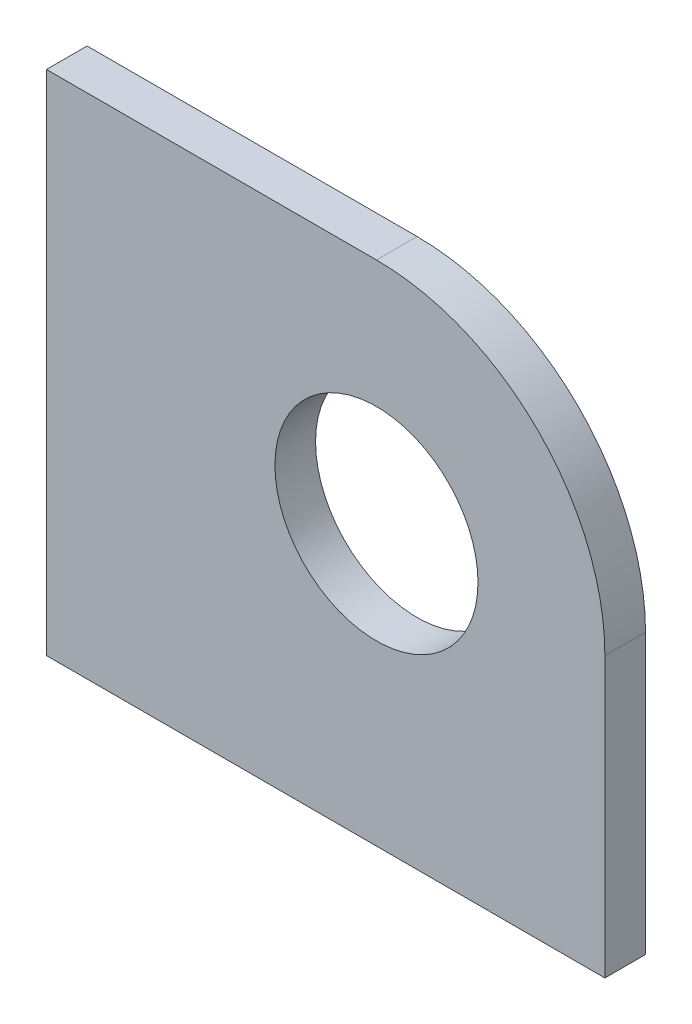
from build123d import *

# Parameters (mm, degrees)
SKETCH1_R           = 20
BOSS_EXTRUDE1_DEPTH = 8


with BuildPart() as part:
    # Sketch1 → Boss-Extrude1 (new body)
    with BuildSketch(Plane.XY):
        with BuildLine():
            Line((0, 0), (110, 0))
            Line((110, 0), (110, 55))
            ThreePointArc((110, 55), (96.819805153, 86.819805153), (65, 100))
            Line((65, 100), (0, 100))
            Line((0, 100), (0, 0))
        make_face()
        with Locations((65, 55)):
            Circle(SKETCH1_R, mode=Mode.SUBTRACT)
    extrude(amount=BOSS_EXTRUDE1_DEPTH)


solid = part.part
